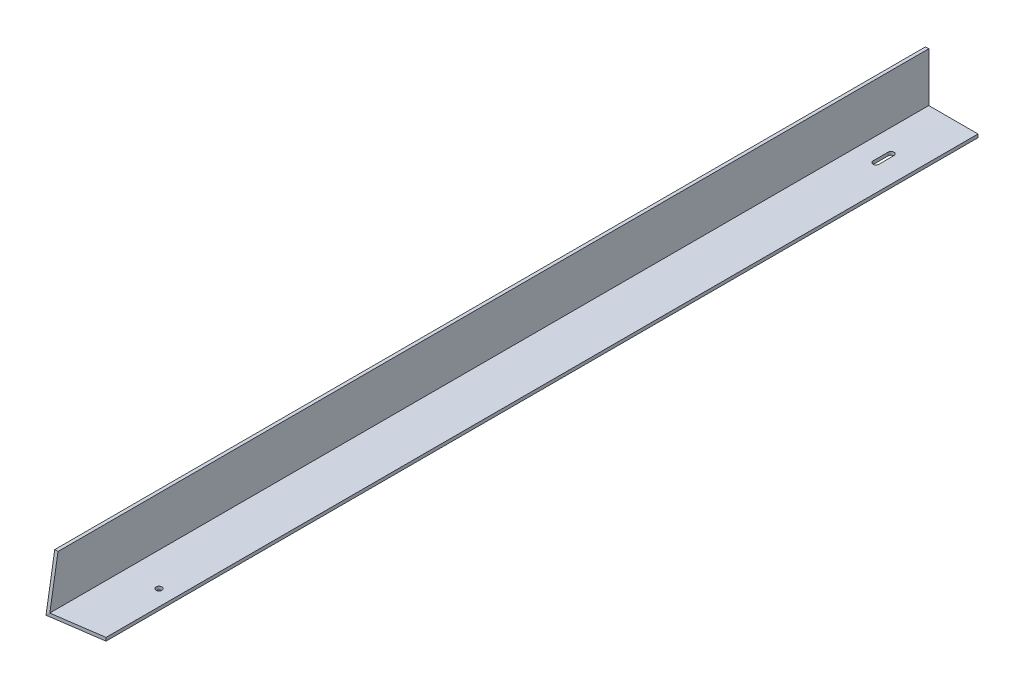
from build123d import *

# Parameters (mm, degrees)
BOSS_EXTRUDE1_DEPTH = 1063.8155
CUT_EXTRUDE1_DEPTH  = 150
SKETCH3_R           = 7.14375
CUT_EXTRUDE2_DEPTH  = 250


with BuildPart() as part:
    # Sketch1 → Boss-Extrude1 (new, symmetric)
    with BuildSketch(Plane.XY):
        Polygon((0, 127), (0, 0), (127, 0), (127, 7.9375), (7.9375, 7.9375), (7.9375, 127), align=None)
    extrude(amount=BOSS_EXTRUDE1_DEPTH, both=True)

    # Sketch2 → Cut-Extrude1 (cut)
    with BuildSketch(Plane.ZY):
        Polygon((1063.8155, 0), (1042.676904036, 127), (1063.8155, 127), align=None)
    extrude(amount=-CUT_EXTRUDE1_DEPTH, mode=Mode.SUBTRACT)

    # Sketch3 → Cut-Extrude2 (cut, symmetric)
    with BuildSketch(Plane(origin=(0, 7.9375, 0), x_dir=(1, 0, 0), z_dir=(0, 1, 0))):
        with Locations(Location((88.9, -879.2845, 0), (0, 0, 270))):
            Circle(SKETCH3_R)
        Polygon((0, -1063.8155), (127, -1063.8155), (127, -1045.559770079), align=None)
        with BuildLine():
            Line((70.64375, 916.97175), (70.64375, 880.45925))
            ThreePointArc((70.64375, 880.45925), (63.5, 873.3155), (56.35625, 880.45925))
            Line((56.35625, 880.45925), (56.35625, 916.97175))
            ThreePointArc((56.35625, 916.97175), (63.5, 924.1155), (70.64375, 916.97175))
        make_face()
    extrude(amount=CUT_EXTRUDE2_DEPTH, both=True, mode=Mode.SUBTRACT)


solid = part.part
